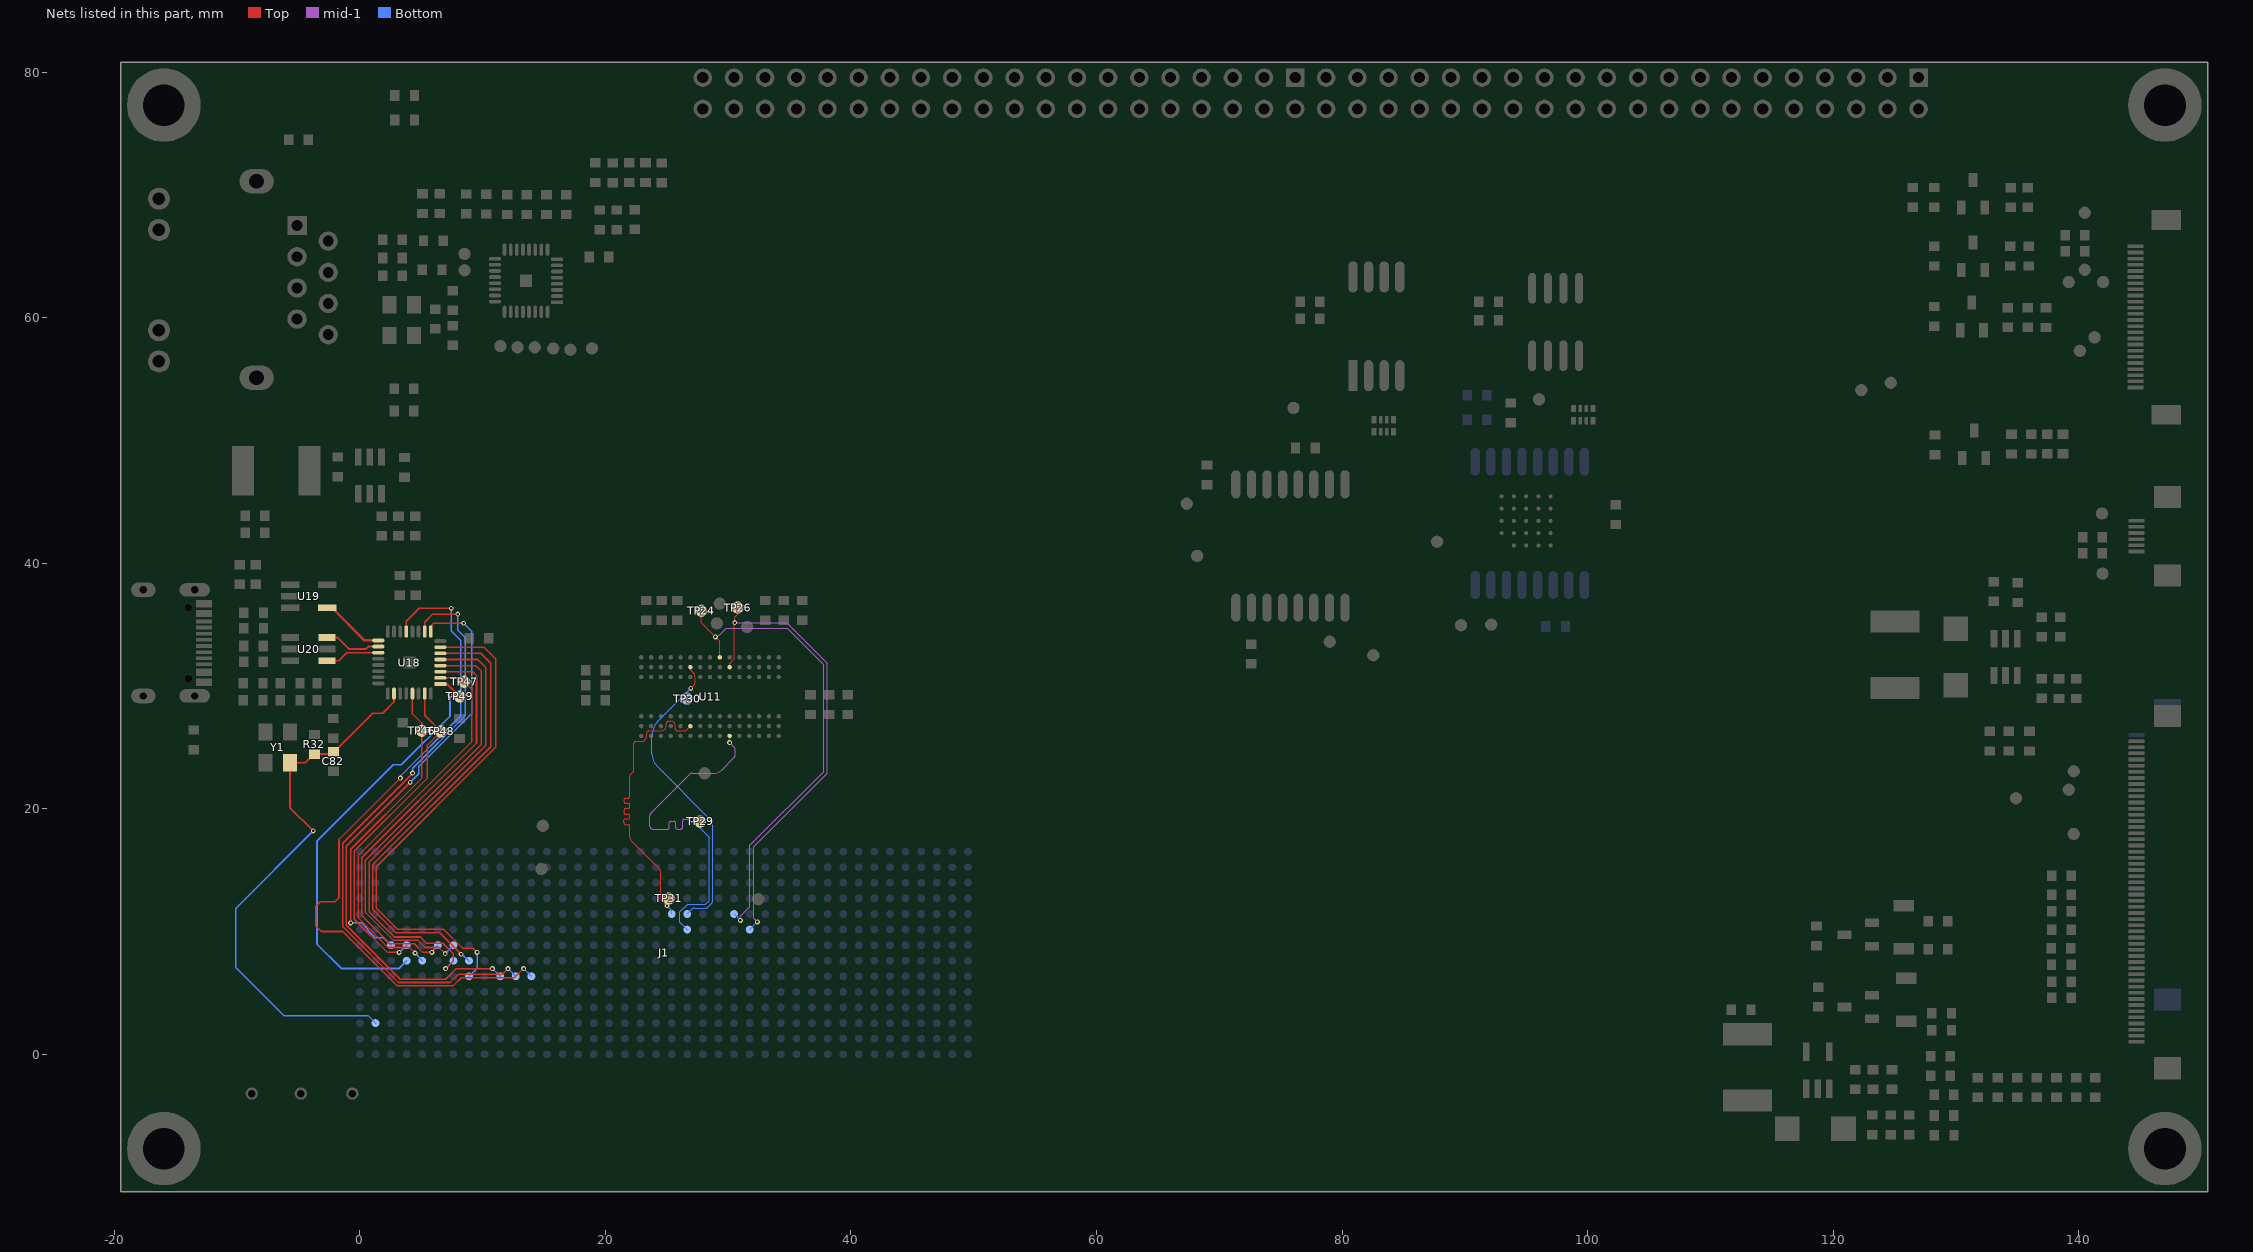
[diagram p0: the nets of this part, all layers, seen from the top]
# Altium PCB MISC105414.PcbDoc (part 11 of 11)
Units mm, origin at the board's own origin, x right, y up, seen from the top; angles counter-clockwise.
Board outline 170 x 92 mm, 6 copper layers (Top, GND, mid-1, mid-2, mid-3, Bottom), stack 1.231 mm thick; 238 components, 304 nets, 1456 pads, 1258 vias.
Unrouted connection lines stored in the file: 57.

## Via types
v1: diameter 0.4, hole 0.2, Top to Bottom, tented top, 618 vias
v2: diameter 0.5, hole 0.3, Top to Bottom, tented top, 522 vias
v3: diameter 0.5, hole 0.3, Top to Bottom, 41 vias
v4: diameter 1, hole 0.5, Top to Bottom, tented top, 36 vias
v5: diameter 0.7, hole 0.4, Top to Bottom, tented top, 34 vias
v6: diameter 1.3, hole 1.3, Top to Bottom, tented top, 3 vias
v7: diameter 4, hole 4, Top to Bottom, tented top, 2 vias
v8: diameter 3.3, hole 3.3, Top to Bottom, tented top, 2 vias

## Nets (pads, with @x,y where several pads share a name; then routed paths per layer and width w, separated by ;. In a path a pad name is that pad's centre, name@x,y a point inside that pad or via, vN(x,y) a via of type N, cw(c..) or ccw(c..) an arc to the next point about the centre after c; other vN are vias at no path point) (continued)
SDR_DQM1: J1.G19 TP29.1 U11.K1 | length 28.5
  Top w0.1: v1(30.11,25.389) 30.12,25.399 U11.K1@30.12,25.933
  mid-1 w0.1: v1(27.026,19.096) 26.984,19.138 26.399,19.138 ccw(c26.399,19.022) 26.283,19.022 26.283,18.489 cw(c26.143,18.489) 26.143,18.349 25.858,18.349 cw(c25.858,18.487) 25.72,18.487 25.72,18.809 ccw(c25.546,18.809) 25.546,18.983 25.33,18.983 ccw(c25.33,18.861) 25.209,18.861 25.209,18.46 cw(c25.098,18.46) 25.098,18.349 23.845,18.349 cw(c23.845,18.569) 23.626,18.569 23.626,19.438 cw(c23.91,19.438) 23.709,19.639 25.197,21.127 25.197,21.14 26.86,22.803 cw(c27.08,22.583) 27.08,22.894 28.828,22.894 ccw(c28.828,23.783) 29.456,23.154 30.494,24.192 ccw(c30.308,24.378) 30.571,24.378 30.571,24.796 ccw(c30.253,24.796) 30.478,25.021 v1(30.11,25.389)
  Bottom w0.1: J1.G19@26.67,10.16 26.067,10.763 26.067,11.593 26.69,12.216 28.152,12.216 28.438,12.502 28.438,17.684 v1(27.026,19.096)
SDR_DQM2: J1.H19 TP30.1 U11.F8 | length 25
  Top w0.1: U11.F8@26.92,31.533 26.92,31.393 ccw(c27.136,31.393) 26.984,31.24 27.184,31.039 cw(c26.905,30.76) 27.3,30.76 27.3,30.283 cw(c26.98,30.283) 27.206,30.056 v1(26.95,29.8)
  Bottom w0.1: J1.H19@26.67,11.43 27.081,11.841 cw(c27.261,11.66) 27.261,11.915 28.203,11.915 ccw(c28.203,12.091) 28.327,11.967 28.653,12.293 ccw(c28.449,12.497) 28.738,12.497 28.738,18.565 ccw(c27.831,18.565) 28.472,19.206 24.207,23.471 cw(c25.207,24.471) 23.792,24.471 23.792,25.927 cw(c25.52,25.927) 24.298,27.148 26.384,29.234 v1(26.95,29.8)
SDR_DQM3: J1.H20 TP31.1 U11.F2 | length 24.1
  Top w0.1: v1(25.015,12.096) 24.562,12.549 cw(c24.71,12.698) 24.5,12.698 24.5,14.834 ccw(c24.081,14.834) 24.377,15.131 22.095,17.413 cw(c22.397,17.714) 21.971,17.714 21.971,18.592 ccw(c21.854,18.592) 21.854,18.708 21.675,18.708 cw(c21.675,18.896) 21.488,18.896 21.488,19.057 cw(c21.603,19.057) 21.603,19.172 21.847,19.172 ccw(c21.847,19.296) 21.971,19.296 21.971,19.457 ccw(c21.869,19.457) 21.869,19.558 21.627,19.558 cw(c21.627,19.671) 21.515,19.671 21.515,19.894 cw(c21.645,19.894) 21.645,20.025 21.869,20.025 ccw(c21.869,20.126) 21.971,20.126 21.971,20.314 ccw(c21.846,20.314) 21.846,20.438 21.637,20.438 cw(c21.637,20.553) 21.522,20.553 21.522,20.768 cw(c21.614,20.768) 21.614,20.86 21.84,20.86 ccw(c21.84,20.991) 21.971,20.991 21.971,22.662 cw(c22.115,22.662) 22.013,22.765 22.293,23.044 ccw(c22.229,23.108) 22.319,23.108 22.319,25.343 cw(c22.489,25.343) 22.489,25.513 23.066,25.513 ccw(c23.066,25.652) 23.164,25.554 23.257,25.647 ccw(c23.032,25.872) 23.35,25.872 23.35,26.157 cw(c23.543,26.157) 23.543,26.35 24.57,26.35 ccw(c24.57,26.73) 24.95,26.73 24.95,26.927 cw(c25.149,26.927) 25.149,27.126 25.317,27.126 cw(c25.317,26.737) 25.706,26.737 25.706,26.497 ccw(c25.853,26.497) 25.853,26.35 26.497,26.35 ccw(c26.497,26.447) 26.566,26.378 U11.F2@26.92,26.733
  Bottom w0.1: v1(25.015,12.096) 25.4,11.711 J1.H20@25.4,11.43
SDR_RAS: J1.H16 TP24.1 U11.J9 | length 39.1
  Top w0.1: TP24.1@27.81,36.126 27.81,35.15 v1(28.964,33.995) 29.32,33.64 U11.J9@29.32,32.333
  mid-1 w0.1: v1(28.964,33.995) 29.231,34.126 29.266,34.133 29.83,34.697 34.8,34.697 37.772,31.725 37.772,23.025 31.769,17.022 31.769,12.027 31.001,11.259 v1(31.001,10.909)
  Bottom w0.1: J1.H16@30.48,11.43 v1(31.001,10.909)
SDR_WE: J1.G15 TP26.1 U11.K8 | length 38.6
  Top w0.1: U11.K8@30.12,31.533 30.12,31.822 30.503,32.205 30.503,35.132 v1(30.532,35.162) 30.536,35.162 30.536,35.61 30.767,35.841 30.767,36.392 TP26.1@30.77,36.392
  mid-1 w0.1: v1(30.532,35.162) 34.761,35.162 38.072,31.85 38.072,22.9 32.07,16.898 32.07,11.099 v1(32.381,10.788)
  Bottom w0.1: J1.G15@31.75,10.16 v1(32.381,10.788)
ULPI_CLK: J1.E37 TP49.1 U18.1 | length 36.3
  Top w0.15: U18.1@6.558,30.159 7.129,30.159 TP49.1@8.14,29.149
  Top w0.2: v1(7.343,29.234) TP49.1@8.14,29.149
  Bottom w0.15: J1.E37@3.81,7.62 3.19,7 -1.518,7 -3.5,8.982 -3.5,17.35 2.732,23.582 3.369,23.582 7.343,27.556 v1(7.343,29.234)
ULPI_D0: J1.F35 U18.3 | length 34.2
  Top w0.127: v1(5.857,8.3) 5.134,8.3 4.434,9 2.45,9 0.15,11.3 0.15,16 9.5,25.35 9.5,30.85 9.19,31.16 U18.3@6.558,31.16
  Bottom w0.127: v1(5.857,8.3) J1.F35@6.35,8.89
ULPI_D1: J1.F34 U18.4 | length 35.9
  Top w0.127: U18.4@6.558,31.66 9.44,31.66 9.9,31.2 9.9,25.25 0.45,15.8 0.45,11.55 2.7,9.3 4.7,9.3 5.3,8.7 6.45,8.7 v1(6.95,8.2)
  Bottom w0.127: v1(6.95,8.2) J1.F34@7.62,8.89
ULPI_D2: J1.E34 U18.5 | length 38.4
  Top w0.127: U18.5@6.558,32.16 9.6,32.16 10.25,31.51 10.25,25.15 0.75,15.65 0.75,11.609 2.805,9.554 4.923,9.554 5.427,9.05 6.75,9.05 7.62,8.18 7.62,7.62 v1(6.985,6.985)
  Bottom w0.127: v1(6.985,6.985) J1.E34@7.62,7.62
ULPI_D3: J1.E33 U18.6 | length 38
  Top w0.127: U18.6@6.558,32.66 9.85,32.66 10.65,31.86 10.65,25.05 1.05,15.45 1.05,11.8 2.95,9.9 6.5,9.9 v1(8.25,8.15)
  Bottom w0.127: v1(8.25,8.15) J1.E33@8.89,7.62
ULPI_D4: J1.D33 U18.7 | length 41.1
  Top w0.127: U18.7@6.558,33.16 10.1,33.16 11.05,32.21 11.05,25 1.336,15.286 1.336,11.914 3.05,10.2 6.8,10.2 8.35,8.65 9.2,8.65 v1(9.55,8.3)
  Bottom w0.127: J1.D33@8.89,6.35 9.55,7.01 v1(9.55,8.3)
ULPI_D5: J1.D31 U18.9 | length 47.3
  Top w0.127: v1(4.1,22.15) -1.114,16.936 -1.114,10.513 3.289,6.111 6.985,6.111 7.859,6.985 v1(10.795,6.985) ; U18.9@5.78,34.438 5.78,34.874 6.02,35.114 v1(8.446,35.114)
  Bottom w0.127: v1(4.1,22.15) 4.803,22.853 4.803,23.439 9.1,27.735 9.1,34.46 v1(8.446,35.114) ; v1(10.795,6.985) J1.D31@11.43,6.35
ULPI_D6: J1.D30 U18.10 | length 50.3
  Top w0.127: v1(4.3,22.9) -1.4,17.2 -1.4,10.4 3.151,5.849 7.349,5.849 8.023,6.523 11.603,6.523 v1(12.065,6.985) ; U18.10@5.28,34.438 5.28,35.201 5.938,35.858 v1(7.974,35.858)
  Bottom w0.127: v1(4.3,22.9) 4.3,23.295 8.6,27.595 8.6,33.934 7.974,34.56 v1(7.974,35.858) ; v1(12.065,6.985) J1.D30@12.7,6.35
ULPI_D7: J1.D29 U18.13 | length 57.2
  Top w0.127: v1(3.3,22.5) -1.7,17.5 -1.7,12.746 -2.021,12.425 -3.225,12.425 -3.6,12.05 -3.6,10.45 -3.15,10 -1.4,10 3.005,5.595 7.621,5.595 8.258,6.232 12.582,6.232 v1(13.335,6.985) ; U18.13@3.78,34.438 3.78,35.28 4.827,36.327 v1(7.442,36.327)
  Bottom w0.127: v1(3.3,22.5) 3.222,22.578 8.213,27.57 8.213,33.706 7.442,34.478 v1(7.442,36.327) ; v1(13.335,6.985) J1.D29@13.97,6.35
ULPI_DIR: J1.F37 TP48.1 U18.31 | length 27.5
  Top w0.127: v1(3.2,8.3) 2.25,8.3 -0.45,11 -0.45,16.55 5.5,22.5 5.5,25.2 TP48.1@6.6,26.3 5.28,27.62 U18.31@5.28,29.382
  Bottom w0.127: v1(3.2,8.3) J1.F37@3.81,8.89
ULPI_NXT: J1.E36 TP47.1 U18.2 | length 32.1
  Top w0.127: v1(4.5,8.25) 4.05,8.7 2.3,8.7 -0.15,11.15 -0.15,16.2 9.094,25.444 9.094,29.756 TP47.1@8.5,30.35 8.433,30.437 8.21,30.66 U18.2@6.558,30.66
  Bottom w0.127: v1(4.5,8.25) J1.E36@5.08,7.62
ULPI_STP: J1.F38 TP46.1 U18.29 | length 25.5
  Top w0.127: v1(-0.75,10.7) -0.75,16.7 5.05,22.5 TP46.1@5.05,26.35 5.05,26.95 4.28,27.72 U18.29@4.28,29.382
  Bottom w0.127: v1(-0.75,10.7) 0.144,10.7 0.65,10.194 0.65,10.096 1.246,9.5 1.93,9.5 J1.F38@2.54,8.89
USB_N: U18.19 U20.1 | length 4.4
  Top w0.15: U20.1@-2.67,32.06 -1.722,32.06 -1.072,32.71 U18.19@1.502,32.71
USB_P: U18.18 U20.3 | length 4.6
  Top w0.15: U20.3@-2.67,33.96 -1.829,33.96 -0.889,33.02 0.508,33.02 0.698,33.21 U18.18@1.502,33.21
USB_PHY_CLK: C82.1 J1.A39 R32.2 U18.26 Y1.1 | length 44.7
  Top w0.15: v1(-3.8,18.2) -5.7,20.1 Y1.1@-5.7,23.75 -4.451,23.75 -3.751,24.45 -2.15,24.45 C82.1@-2.15,24.65 -2.099,24.65 1.032,27.781 1.854,27.781 2.78,28.707 U18.26@2.78,29.382
  Bottom w0.127: v1(-3.8,18.2) -10.118,11.882 -10.118,7.07 -6.198,3.15 0.66,3.15 J1.A39@1.27,2.54
VBUS_EN: U18.17 U19.4 | length 5.3
  Top w0.2: U19.4@-2.664,36.378 -2.278,36.378 0.39,33.71 U18.17@1.502,33.71
pads on no net: DESIGNATOR1.1 DESIGNATOR2.1 DESIGNATOR3.1 DESIGNATOR4.1 ETH1.7 J1.B1 J1.B36 J1.B37 J1.B40 J1.D1 J1.D34 J1.E9 J1.E12 J1.E13 J1.E16 J1.E21 J1.E22 J1.E24 J1.E25 J1.E27 J1.E28 J1.E30 J1.E31 J1.F1 J1.F7 J1.F10 J1.F11 J1.F14 J1.F19 J1.F22 J1.F23 J1.F25 J1.F26 J1.F28 J1.F29 J1.F31 J1.F32 J1.G2 J1.G3 J1.G9 J1.G10 J1.G12 J1.G13 J1.H1 J1.H2 J1.H4 J1.H5 J1.H7 J1.H8 J1.H10 J1.H11 J1.J2 J1.J3 J1.J15 J1.J39 J1.K1 J1.K4 J1.K5 J1.K37 J1.K40 J1.L1 J1.L32 J1.L33 J1.M18 J1.M26 J1.M27 J1.M30 J1.M31 J1.M34 J1.M35 J1.M38 J1.M39 J1.Y34 J1.Y35 J1.Y38 J1.Y39 J1.Z1 J1.Z32 J1.Z33 J1.Z36 J1.Z37 J1.Z40 J2.45 J2.49 J2.50 J3.35 J3.37 J3.38 J3.39 J3.40 J4.1 J5.14 J5.16 J5.18 U9.A2 U9.A5 U9.B1 U9.B5 U9.C2 U9.C5 U11.E3 U11.E7 U11.K2 U11.K3 U11.R1 U13.3 U17.13 U17.15 U18.12 U18.15 U18.16 USB1. USB1.3 USB1.9
copper on no net:
  other v1: 39.675,31.45
  other v4: -15.97,-10.09 147.03,-10.09 -17.667,-9.387 -14.273,-9.387 145.333,-9.387 148.727,-9.387 -18.37,-7.69 -13.57,-7.69 144.63,-7.69 149.43,-7.69 -17.667,-5.993 -14.273,-5.993 145.333,-5.993 148.727,-5.993 -15.97,-5.29 -15.97,-5.29 147.03,-5.29 147.03,-5.29 -15.97,74.91 147.03,74.91 -17.667,75.613 -14.273,75.613 145.333,75.613 148.727,75.613 -18.37,77.31 -13.57,77.31 144.63,77.31 149.43,77.31 -17.667,79.007 -14.273,79.007 145.333,79.007 148.727,79.007 -15.97,79.71 -15.97,79.71 147.03,79.71 147.03,79.71
  other v6: 51.841,8.255 -2.438,11.303
  other v7: -6.47,10.81 56.03,10.81
  other v8: -11.465,57.345 -11.465,68.775

## Polygon pours and split planes (outlines as drawn)
GND on mid-1 "NONET_L03_P010" (solid, remove dead copper, shelved, pour order 10): -19.47,80.81 150.53,80.81 150.53,-11.19 -19.47,-11.19
+5V_USB on mid-1 "NONET_L03_P000" (solid, shelved, pour order 0): -10.725,38.4 -12.275,36.85 -12.275,30.825 -12.225,30.825 -11.225,29.825 -11.175,29.875 -9.325,29.875 -8.55,30.65 -8.55,38.2 -8.75,38.4 -10.65,38.4
+1_8V on mid-3 "NONET_L05_P005" (solid, shelved, pour order 5): 75,80.6 75,74.2 72.9,72.1 30.1,72.1 28,70 28,57.3 11.9,41.2 4.7,41.2 3.931,40.431 3.931,38.197 8.703,38.197 10.65,36.25 10.65,19.85 4.3,13.5 -2.7,13.5 -3.4,12.8 -3.4,9.5 -2,8.1 0.5,8.1 41.95,8.1 44.126,10.276 44.126,29.226 46.1,31.2 99.3,31.2 104.6,36.5 104.6,66.1 103.3,67.4 85.1,67.4 80,72.5 80,80.4 79.8,80.6
+12V on mid-3 "NONET_L05_P006" (solid, shelved, pour order 6): 7.6,44.3 1.8,44.3 0.8,43.3 0.8,30.4 -11.1,18.5 -11.1,6.1 -8.2,3.2 6.7,3.2 7.7,4.2 7.7,6.3 6.1,7.9 -2.9,7.9 -3.9,8.9 -3.9,13.2 -2.8,14.3 4.5,14.3 6.3,16.1 6.3,23.4 2.9,26.8 2.9,40.2 4.3,41.6 7.7,41.6 8,41.9 8,43.9
GND on mid-3 "NONET_L05_P011" (solid, remove dead copper, shelved, pour order 11): -19.47,80.81 150.53,80.81 150.53,-11.19 -19.47,-11.19
+3_3V on mid-3 "NONET_L05_P007" (solid, shelved, pour order 7): 28.4,80.6 24.6,80.6 21.662,77.662 21.662,62.962 9.675,50.975 -15.025,50.975 -17.8,48.2 -17.8,-2.8 -10.6,-10 133.9,-10 135.2,-8.7 135.2,-4.45 134.85,-4.1 122,-4.1 121.4,-3.5 121.4,7.7 129.3,15.6 129.3,80 128.5,80.8 118.2,80.8 115.1,77.7 115.1,26.5 87.3,-1.3 -5.8,-1.3 -12.1,5 -12.1,19 -4.6,26.5 -4.6,33.375 -12.6,41.375 -12.6,44.375 -11.6,45.375 15.2,45.375 27.5,57.675 27.5,71.35 29.3,73.15 29.3,79.7
+1_8V_ETH on mid-3 "NONET_L05_P003" (solid, shelved, pour order 3): 21.5,68.6 12.6,77.5 3.2,77.5 1.2,75.5 1.2,54.3 3.7,51.8 8.1,51.8 20.5,64.2 21.5,64.2
LCD_DVDD on mid-3 "NONET_L05_P004" (solid, remove dead copper, shelved, pour order 4): 140.5,44.9 133.2,37.6 133.2,3.6 130.3,0.7 125.8,0.7 125.8,-3.6 139.7,-3.6 144.215,0.915 144.215,44.285 143.6,44.9
+5V on mid-3 "NONET_L05_P002" (solid, shelved, pour order 2): -12.25,41.45 -1.2,30.4 -0.2,30.4 0.5,31.1 0.5,39.6 -4.3,44.4 -12.25,44.4
+1_8V_ULPI on mid-3 "NONET_L05_P001" (solid, shelved, pour order 1): 3,37.5 3,27.5 3.5,27 7.3,27 9.4,29.1 9.4,36.5 7.9,38 3.5,38
GND on Top "NONET_L01_P008" (solid, remove dead copper, shelved, pour order 8): -19.47,80.81 150.53,80.81 150.53,-11.19 -19.47,-11.19
GND on GND "NONET_L02_P009" (solid, remove dead copper, shelved, pour order 9): -19.47,80.81 150.53,80.81 150.53,-11.19 -19.47,-11.19
GND on Bottom "NONET_L06_P012" (solid, remove dead copper, shelved, pour order 12): -19.47,80.81 150.53,80.81 150.53,-11.19 -19.47,-11.19
GND on mid-2 "NONET_L04_P013" (solid, remove dead copper, shelved, pour order 13): -19.47,80.81 150.53,80.81 150.53,-11.19 -19.47,-11.19

## Keep-outs
Keep-Out Layer:
  the board outline again, w0.2

## Other copper
Top:
  rectangle net +1_8V: 22,68.3 29.4,69.8
  rectangle net +1_8V_ETH: 19.1,65.9 22.9,67.5
  region net LCD_LED-: 147.95,24.075 148.625,23.4 149.175,23.4 149.2,23.425 149.2,24.7 149.075,24.825 148.425,24.825 147.95,24.35 147.95,24.05
  pour cut-out: -19.47,71.06 -0.882,71.06 -0.882,55.06 -19.47,55.06
  region net +12V: 3.8,48 4.3,48 5.7,46.6 5.7,42.7 5.9,42.5 7.5,42.5 7.7,42.7 7.7,46.8 4.5,50 3.1,50 3.1,48.1 3.2,48 3.3,48.1 4.2,48.1
  region net NETD1_1: 132.9,31.4 132.6,31.1 123.5,31.1 122.8,30.4 122.8,29.3 123.3,28.8 123.5,29 132.6,29 133.3,29.7 133.3,31.4
  region net +3_3V: 133.5,37.2 132.5,37.2 131.2,38.5 123.9,38.5 122.7,37.3 122.7,34.8 123.1,34.4 126.7,34.4 128.5,36.2 131.2,36.2 132.4,35 132.4,33.7 132.8,33.3 133.3,33.3 133.3,36.7 133.1,36.9
  region net LCD_LED-: 135.4,31 135.2,31.2 134.9,31.2 134.9,30.1 135.2,29.8 136.7,29.8 137.4,30.5 137.4,31
  region net +10_4V_AVDD: 128.35,-6.15 122.45,-6.15 121.8,-5.5 120.1,-5.5 120.1,-7.1 121.4,-8.4 127.4,-8.4 128.565,-7.235 128.565,-6.365 128.5,-6.3
  region net NETC12_2: 111.9,-2.1 111,-3 111.1,-3.1 111.1,-5.5 112.8,-7.2 117,-7.2 117.9,-6.3 117.9,-2.2 117.7,-2.2 117.6,-2.1
  region net +3_3V: 112.9,1.3 113.5,0.7 116.3,0.7 117.5,-0.5 118.1,-0.5 118.2,-0.4 118.2,2.2 115.9,4.5 112.912,4.5 112.912,3.912 112.9,3.9
  region net NETC12_2: 119.4,6.1 119.1,6.4 116.8,6.4 116.8,4.7 117.1,4.4 117.5,4.4 117.9,4.8 117.9,5.1 118.1,5.3 119.3,5.3 119.4,5.4
  region net +1_8V: 33.32,30.733 35.153,28.9 40.1,28.9 40.3,29.1 40.3,30.5 40.1,30.7 36.7,30.7 36.1,30.1 35.1,30.1 34.467,30.733 34.12,30.733
  region net +1_8V: 32.6,35.7 32.6,34.2 31.72,33.32 31.72,32.98 31.8,32.9 36.6,32.9 37.8,34.1 37.8,35.759 32.659,35.759
  region net +1_8V: 26.3,35.8 21.2,35.8 19.593,34.193 19.593,28.507 19.7,28.4 20.4,28.4 21.2,29.2 21.2,33.1 22.4,34.3 27,34.3 27,35.1
  region net +3_3V: 24.2,73.6 24.6,74 26.9,74 27.3,73.6 27.3,72.4 27,72.1 26.982,72.118 24.582,72.118 24.2,72.5 24.2,73
  region net +1_8V_ULPI: 2.9,37.7 2.4,37.2 2.4,36.3 2.9,35.8 3.8,35.8 4.8,36.8 4.8,37.6 4.7,37.7
  region net +1_8V: 4,38.7 4.2,38.5 4.215,38.515 5.415,38.515 5.7,38.8 5.7,40.4 5.5,40.6 4.1,40.6 4,40.5
  region net +5V: -3.2,39.7 -3.5,39.4 -3.5,38.1 -3.3,37.9 -0.7,37.9 -0.4,38.2 -0.4,39.4 -0.7,39.7
  region net +5V: -12.4,49.6 -13.7,48.3 -13.7,42.6 -12.8,41.7 -9.3,41.7 -8.7,42.3 -8.7,49.5 -8.8,49.6
  region net NETC76_2: 0.1,48 0.1,50.3 -0.2,50.6 -5,50.6 -5.3,50.3 -5.3,47.7 -4.8,47.2 -3.5,47.2 -3.5,47.3 -2.8,48
  region net +12V: 0.6,48 0.6,49.8 0.8,50 3.9,50 4.8,49.1 4.8,48.744 4.056,48 0.9,48 0.8,48.1
  region net +5V_USB: -13.35,31.35 -13.35,30.825 -11.725,30.825 -11.175,30.275 -10.525,30.275 -10.375,30.425 -10.375,30.75 -11.025,31.4 -13.3,31.4
  region net +5V_USB: -10.2,37.1 -7.745,37.1 -6.8,38.045 -6.8,38.5 -9.7,38.5 -10.2,38 -10.2,37.2
  region net +5V_USB: -11.635,36.195 -11.29,36.54 -11.29,38.31 -10.8,38.8 -4.8,38.8 -4.8,37.9 -8.95,37.9 -11.2,35.65 -13.171,35.65 -13.208,35.687 -13.208,36.195 -12.954,36.195
mid-1:
  pour cut-out: -19.47,71.01 -0.882,71.01 -0.882,55.01 -19.47,55.01
mid-2:
  pour cut-out: -19.495,71.035 -0.907,71.035 -0.907,55.035 -19.495,55.035
mid-3:
  pour cut-out: -19.47,71.06 -0.882,71.06 -0.882,55.06 -19.47,55.06
GND:
  pour cut-out: -19.47,71.06 -0.882,71.06 -0.882,55.06 -19.47,55.06
Bottom:
  pour cut-out: -19.47,71.06 -0.882,71.06 -0.882,55.06 -19.47,55.06
  region net +10_4V_AVDD: 125.8,-5.7 124.9,-6.6 124.9,-7.7 125.2,-8 127,-8 127.3,-7.7 127.3,-6.3 126.7,-5.7

## Silkscreen, mask and mechanical layers (free items; w line width, h text height)
Silkscreen Top:
  lines w0.12: -10.6,36.4 -10.6,28.3 -10.4,28.1 -1,28.1 -1,31 -6.5,31 -7,31.5 -7,37 -10.1,37 -10.6,36.5 ; -17.4,16.9 -17.4,23.7 -17.2,23.9 -12,23.9 -11.7,23.6 -11.7,20.7 -11.5,20.5 -8,20.5 -7.8,20.3 -7.8,16.6 -8.5,16.6 -17.1,16.6 -17.4,16.9